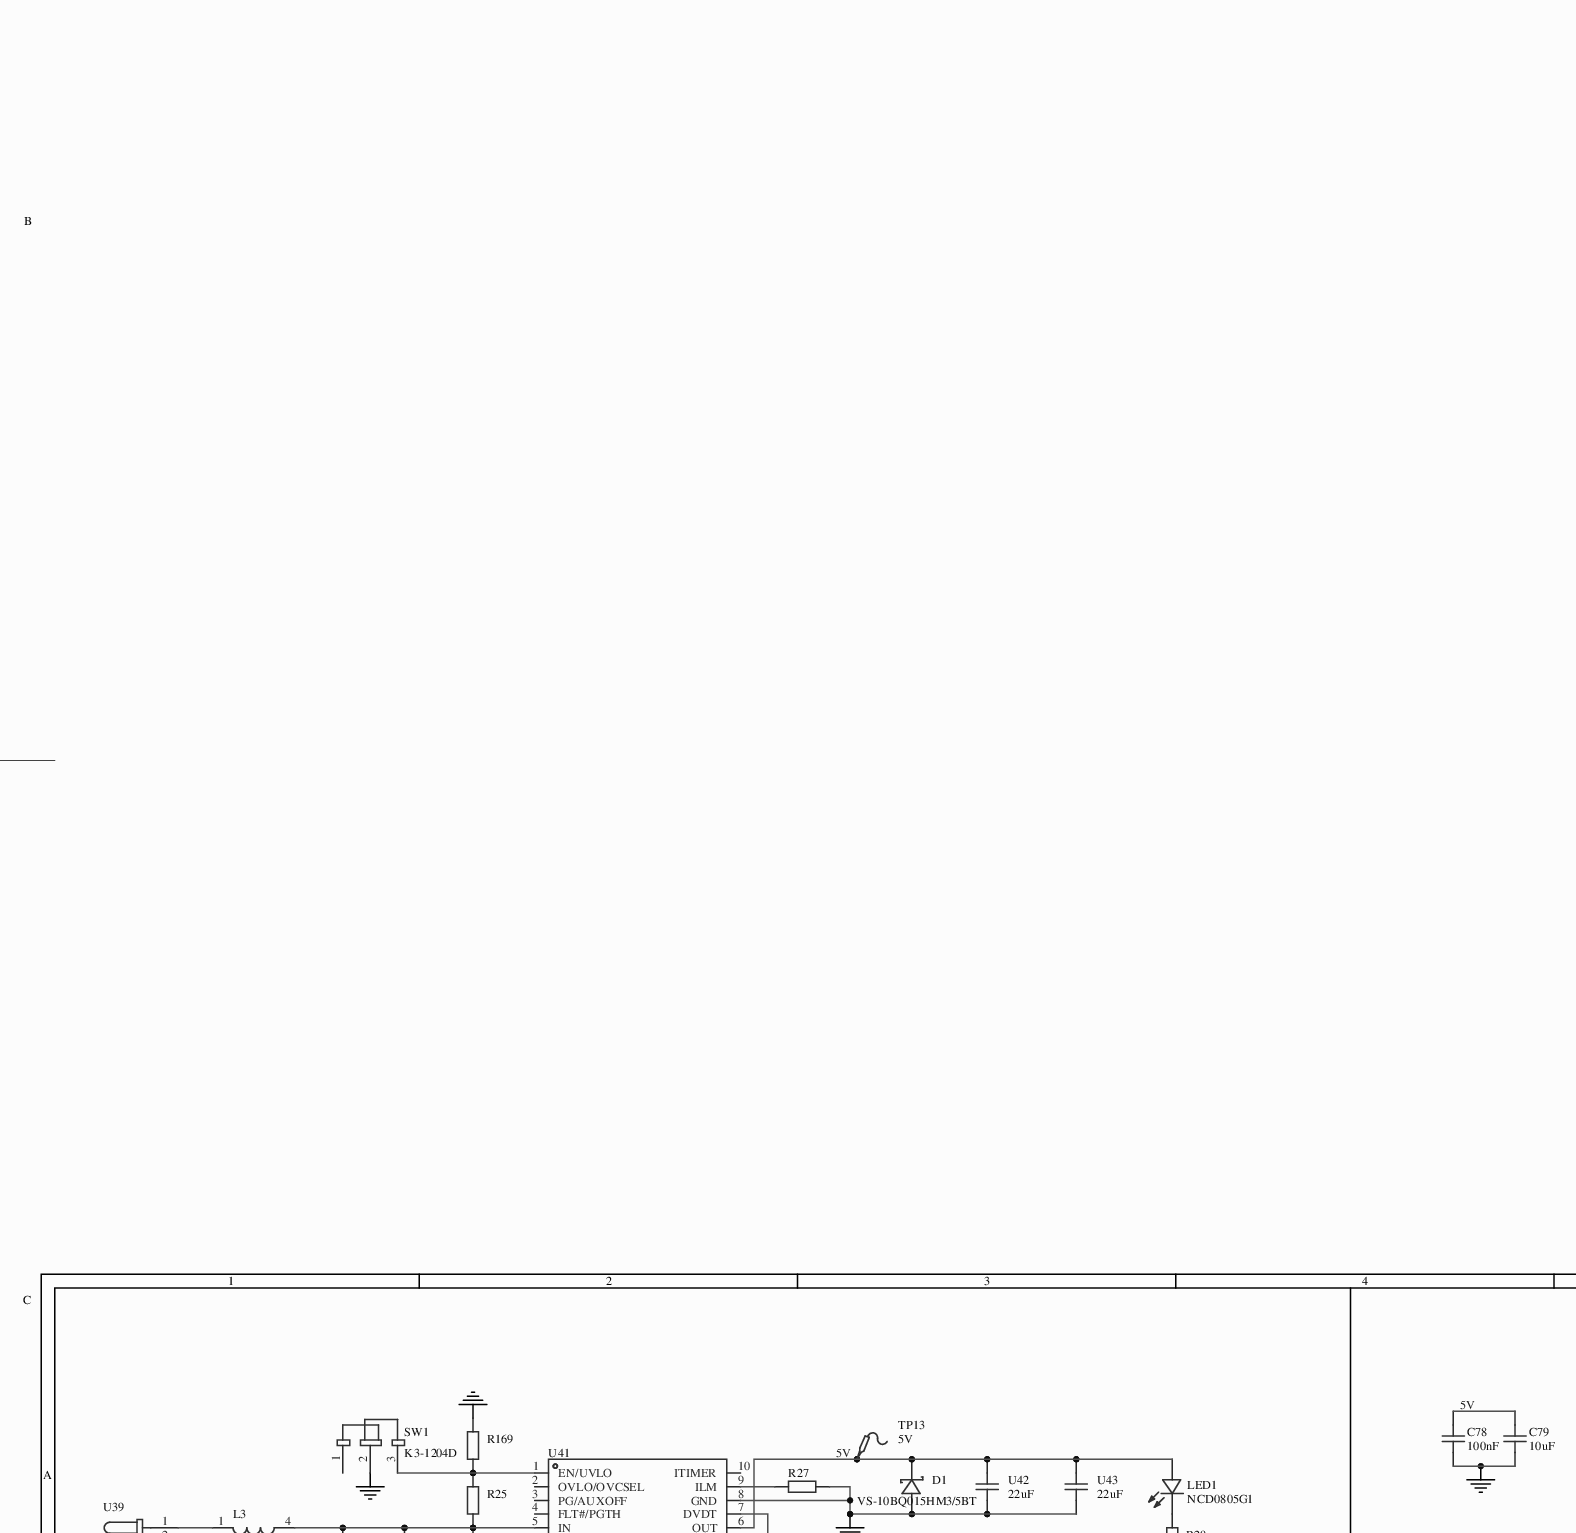
[diagram p0: MISC82799-2.schdoc, centre column 1 of 4]
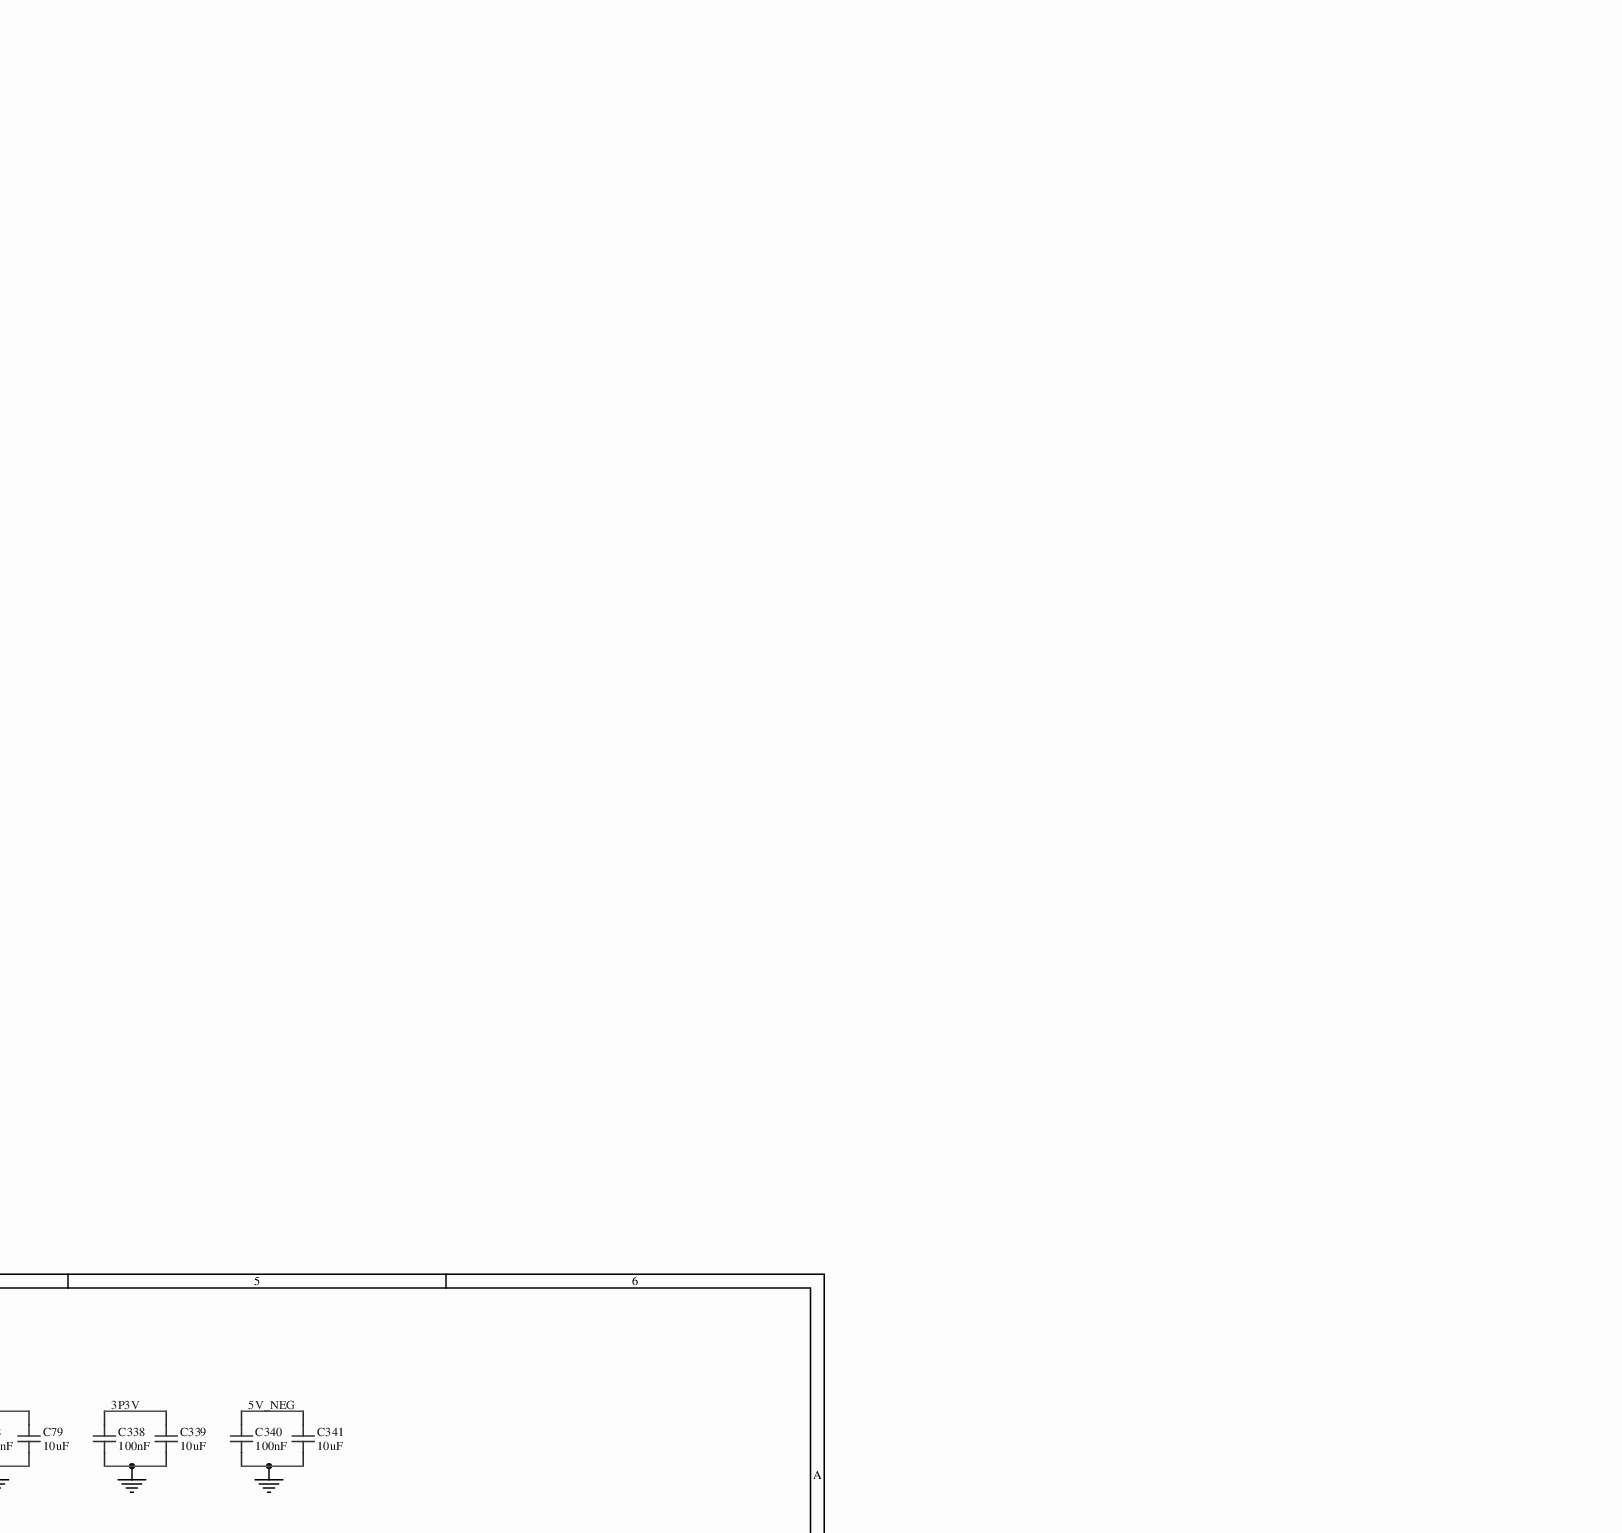
[diagram p1: MISC82799-2.schdoc, centre column 2 of 4]
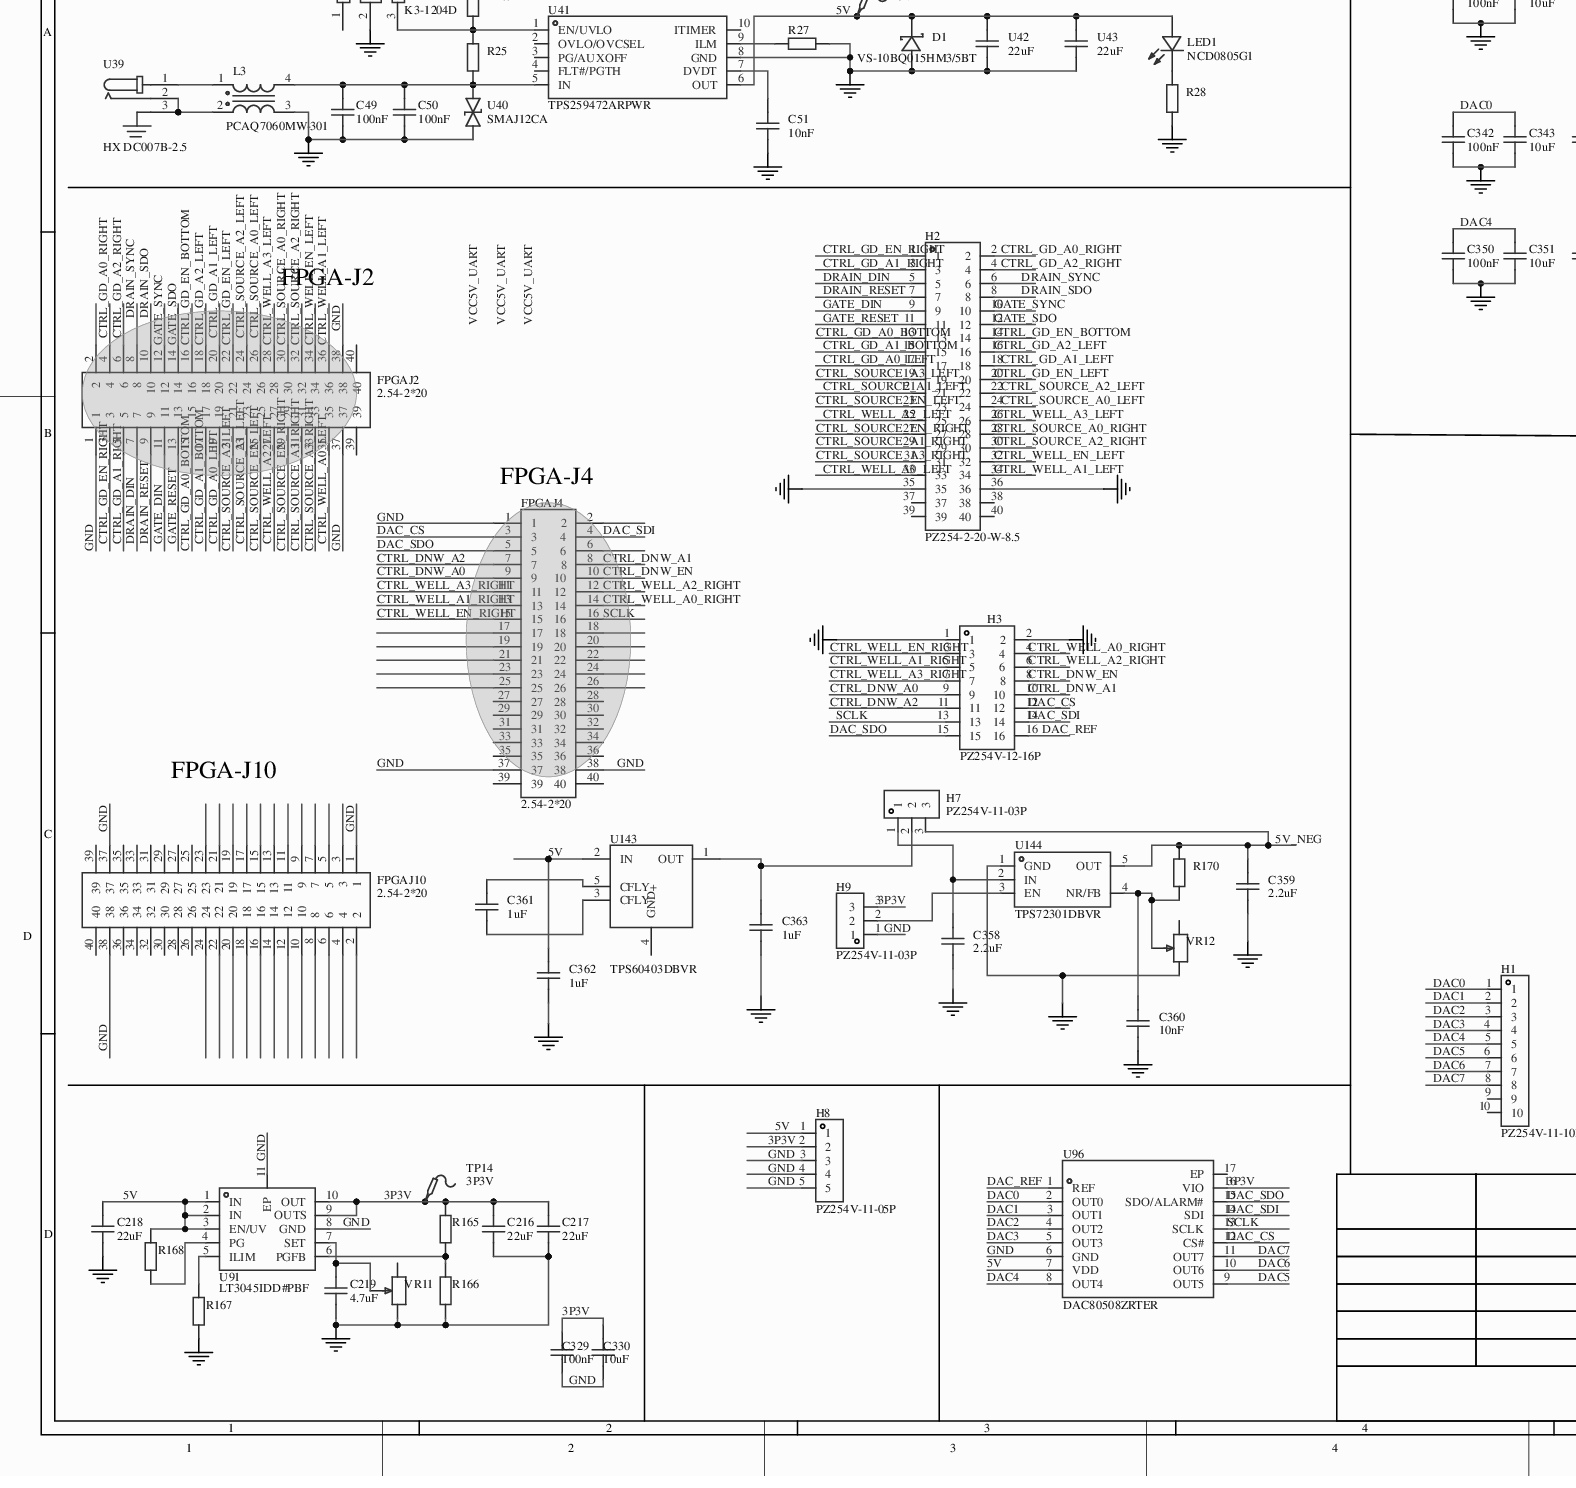
[diagram p2: MISC82799-2.schdoc, bottom column 1 of 4]
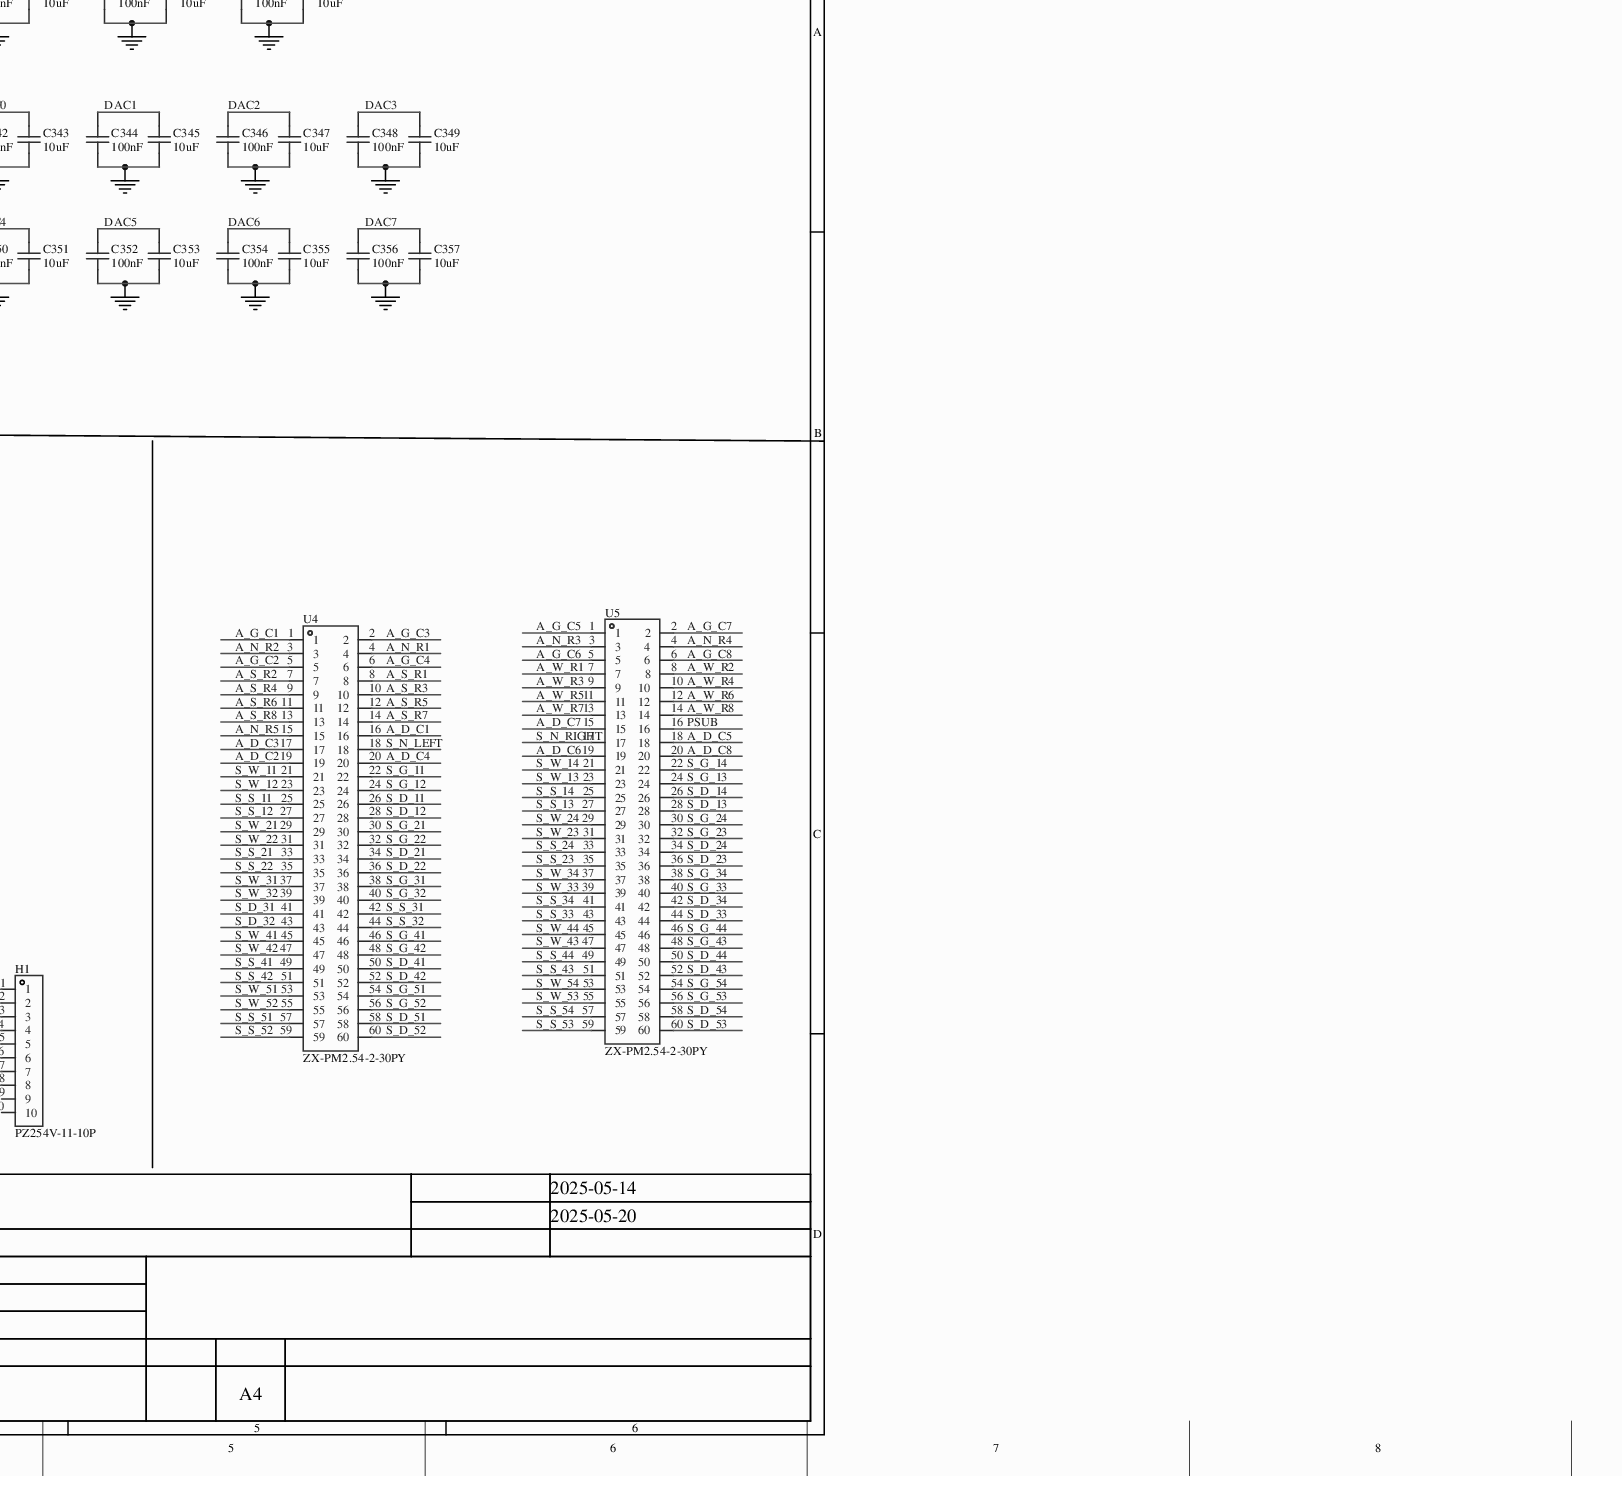
[diagram p3: MISC82799-2.schdoc, bottom column 2 of 4]
# Altium project MISC82799-9.PrjPCB (part 1 of 3)
2 sheets, 95 parts. Net scope: global (net labels, ports and power ports of the same name join across sheets).
Board file: MISC82799.PcbDoc
Sheets:
  MISC82799-2.schdoc
  MISC82799-4.schdoc

## Sheet MISC82799-2.schdoc
size A0; Name: MISC82799; @Page No: 1; @Page Count: 2; @Schematic Name: MISC82799; @Project Name: MISC82799; @Board Name: MISC82799; @Update Date: 2025-05-26; @Create Time: 16:47:34; @Update Time: 16:47:50; @Create Date: 2025-05-26

### Parts
C49  100nF  [C0603]
C50  100nF  [C0603]
C51  10nF  [C0805]
C78  100nF  [C0603]
C79  10uF  [C0603]
C216  22uF  [C0603]
C217  22uF  [C0603]
C218  22uF  [C0603]
C219  4.7uF  [C0603]
C329  100nF  [C0805]
C330  10uF  [C0805]
C338  100nF  [C0603]
C339  10uF  [C0603]
C340  100nF  [C0603]
C341  10uF  [C0603]
C342  100nF  [C0603]
C343  10uF  [C0603]
C344  100nF  [C0603]
C345  10uF  [C0603]
C346  100nF  [C0603]
C347  10uF  [C0603]
C348  100nF  [C0603]
C349  10uF  [C0603]
C350  100nF  [C0603]
C351  10uF  [C0603]
C352  100nF  [C0603]
C353  10uF  [C0603]
C354  100nF  [C0603]
C355  10uF  [C0603]
C356  100nF  [C0603]
C357  10uF  [C0603]
C358  2.2uF  [C0603]
C359  2.2uF  [C0603]
C360  10nF  [C0805]
C361  1uF  [C0603]
C362  1uF  [C0603]
C363  1uF  [C0603]
D1  VS-10BQ015HM3/5BT  [SMB_L4.6-W3.6-LS5.3-RD]
FPGAJ2  2.54-2*20  [HDR-TH_40P-P2.54-V-F-R2-C20-S2.54]
FPGAJ4  2.54-2*20  [HDR-TH_40P-P2.54-V-F-R2-C20-S2.54]
FPGAJ10  2.54-2*20  [HDR-TH_40P-P2.54-V-F-R2-C20-S2.54]
H1  PZ254V-11-10P  [HDR-TH_10P-P2.54-V-M]
H2  PZ254-2-20-W-8.5  [HDR-TH_40P-P2.54-V-F-R2-C20-S2.54]
H3  PZ254V-12-16P  [HDR-TH_16P-P2.54-V-M-R2-C8-S2.54]
H7  PZ254V-11-03P  [HDR-TH_3P-P2.54-V-M]
H8  PZ254V-11-05P  [HDR-TH_5P-P2.54-V-M]
H9  PZ254V-11-03P  [HDR-TH_3P-P2.54-V-M]
L3  PCAQ7060MW-301  [FILTER-SMD_4P-L7.0-W6.0-BL]
LED1  NCD0805G1  [LED0805-R-RD]
R25  (no value)  [R0603]
R27  (no value)  [R0603]
R28  (no value)  [R0603]
R165  (no value)  [R0603]
R166  (no value)  [R0603]
R167  (no value)  [R0603]
R168  (no value)  [R0603]
R169  (no value)  [R0603]
R170  (no value)  [R0603]
SW1  K3-1204D  [SW-TH_K3-1204D]
TP13  5V  [Test-Point-0.5mm]
TP14  3P3V  [Test-Point-0.5mm]
U4  ZX-PM2.54-2-30PY  [HDR-TH_60P-P2.54-V-F-R2-C30-S2.54]
U5  ZX-PM2.54-2-30PY  [HDR-TH_60P-P2.54-V-F-R2-C30-S2.54]
U39  HX DC007B-2.5  [DC-IN-TH_HX-DC007B-2.5]
U40  SMAJ12CA  [SMA_L4.3-W2.7-LS5.1-BI]
U41  TPS259472ARPWR  [VQFN-10_L2.0-W2.0-P0.45-TL]
U42  22uF  [C0805]
U43  22uF  [C0805]
U91  LT3045IDD#PBF  [DFN-10_L3.0-W3.0-P0.50-BL-EP-3]
U96  DAC80508ZRTER  [WQFN-16_L3.0-W3.0-P0.50-TL-EP0.8]
U143  TPS60403DBVR  [SOT-23-5_L3.0-W1.7-P0.95-LS2.8-BR]
U144  TPS72301DBVR  [SOT-23-5_L3.0-W1.7-P0.95-LS2.8-BR]
VR11  (no value)  [RES-ADJ-SMD_3224W]
VR12  (no value)  [RES-ADJ-SMD_3224W]

### Nets
GND: C49.1 C50.1 C51.1 C78.1 C79.1 C216.1 C217.1 C218.1 C219.1 C329.1 C330.1 C338.1 C339.1 C340.1 C341.1 C342.1 C343.1 C344.1 C345.1 C346.1 C347.1 C348.1 C349.1 C350.1 C351.1 C352.1 C353.1 C354.1 C355.1 C356.1 C357.1 C358.1 C359.1 C360.1 C362.1 C363.1 D1.2(A) FPGAJ2.1 FPGAJ2.37 FPGAJ2.38 FPGAJ4.1 FPGAJ4.37 FPGAJ4.38 FPGAJ10.1 FPGAJ10.37 FPGAJ10.38 H2.35 H2.36 H3.1 H3.2 H8.3 H8.4 H8.5 H9.1 L3.3 R27.2 R28.1 R166.1 R167.1 R169.2 SW1.2 U40.1 U41.8(GND) U42.1 U43.1 U91.8(GND) U91.11(EP) U96.6(GND) U144.1(GND) VR11.3 VR12.3
3P3V: C216.2 C217.2 C329.2 C330.2 C338.2 C339.2 H8.2 H9.3 R165.2 TP14.1 U91.9(OUTS) U91.10(OUT) U96.16(VIO)
5V: C78.2 C79.2 C218.2 C362.2 D1.1(C) H8.1 LED1.1(A) R168.2 TP13.1 U41.6(OUT) U42.2 U43.2 U91.1(IN) U91.2(IN) U91.3(EN/UV) U96.7(VDD) U143.2(IN)
5V_NEG: C340.2 C341.2 C359.2 H7.3 R170.2 U144.5(OUT)
A_D_C1: U4.16
A_D_C2: U4.19
A_D_C3: U4.17
A_D_C4: U4.20
A_D_C5: U5.18
A_D_C6: U5.19
A_D_C7: U5.15
A_D_C8: U5.20
A_G_C1: U4.1
A_G_C2: U4.5
A_G_C3: U4.2
A_G_C4: U4.6
A_G_C5: U5.1
A_G_C6: U5.5
A_G_C7: U5.2
A_G_C8: U5.6
A_N_R1: U4.4
A_N_R2: U4.3
A_N_R3: U5.3
A_N_R4: U5.4
A_N_R5: U4.15
A_S_R1: U4.8
A_S_R2: U4.7
A_S_R3: U4.10
A_S_R4: U4.9
A_S_R5: U4.12
A_S_R6: U4.11
A_S_R7: U4.14
A_S_R8: U4.13
A_W_R1: U5.7
A_W_R2: U5.8
A_W_R3: U5.9
A_W_R4: U5.10
A_W_R5: U5.11
A_W_R6: U5.12
A_W_R7: U5.13
A_W_R8: U5.14
CTRL_DNW_A0: FPGAJ4.9 H3.9
CTRL_DNW_A1: FPGAJ4.8 H3.10
CTRL_DNW_A2: FPGAJ4.7 H3.11
CTRL_DNW_EN: FPGAJ4.10 H3.8
CTRL_GD_A0_BOTTOM: FPGAJ2.15 H2.13
CTRL_GD_A0_LEFT: FPGAJ2.19 H2.17
CTRL_GD_A0_RIGHT: FPGAJ2.4 H2.2
CTRL_GD_A1_BOTTOM: FPGAJ2.17 H2.15
CTRL_GD_A1_LEFT: FPGAJ2.20 H2.18
CTRL_GD_A1_RIGHT: FPGAJ2.5 H2.3
CTRL_GD_A2_LEFT: FPGAJ2.18 H2.16
CTRL_GD_A2_RIGHT: FPGAJ2.6 H2.4
CTRL_GD_EN_BOTTOM: FPGAJ2.16 H2.14
CTRL_GD_EN_LEFT: FPGAJ2.22 H2.20
CTRL_GD_EN_RIGHT: FPGAJ2.3 H2.1
CTRL_SOURCE_A0_LEFT: FPGAJ2.26 H2.24
CTRL_SOURCE_A0_RIGHT: FPGAJ2.30 H2.28
CTRL_SOURCE_A1_LEFT: FPGAJ2.23 H2.21
CTRL_SOURCE_A1_RIGHT: FPGAJ2.31 H2.29
CTRL_SOURCE_A2_LEFT: FPGAJ2.24 H2.22
CTRL_SOURCE_A2_RIGHT: FPGAJ2.32 H2.30
CTRL_SOURCE_A3_LEFT: FPGAJ2.21 H2.19
CTRL_SOURCE_A3_RIGHT: FPGAJ2.33 H2.31
CTRL_SOURCE_EN_LEFT: FPGAJ2.25 H2.23
CTRL_SOURCE_EN_RIGHT: FPGAJ2.29 H2.27
CTRL_WELL_A0_LEFT: FPGAJ2.35 H2.33
CTRL_WELL_A0_RIGHT: FPGAJ4.14 H3.4
CTRL_WELL_A1_LEFT: FPGAJ2.36 H2.34
CTRL_WELL_A1_RIGHT: FPGAJ4.13 H3.5
CTRL_WELL_A2_LEFT: FPGAJ2.27 H2.25
CTRL_WELL_A2_RIGHT: FPGAJ4.12 H3.6
CTRL_WELL_A3_LEFT: FPGAJ2.28 H2.26
CTRL_WELL_A3_RIGHT: FPGAJ4.11 H3.7
CTRL_WELL_EN_LEFT: FPGAJ2.34 H2.32
CTRL_WELL_EN_RIGHT: FPGAJ4.15 H3.3
DAC0: C342.2 C343.2 H1.1 U96.2(OUT0)
DAC1: C344.2 C345.2 H1.2 U96.3(OUT1)
DAC2: C346.2 C347.2 H1.3 U96.4(OUT2)
DAC3: C348.2 C349.2 H1.4 U96.5(OUT3)
DAC4: C350.2 C351.2 H1.5 U96.8(OUT4)
DAC5: C352.2 C353.2 H1.6 U96.9(OUT5)
DAC6: C354.2 C355.2 H1.7 U96.10(OUT6)
DAC7: C356.2 C357.2 H1.8 U96.11(OUT7)
DAC_CS: FPGAJ4.3 H3.12 U96.12(CS#)
DAC_REF: H3.16 U96.1(REF)
DAC_SDI: FPGAJ4.4 H3.14 U96.14(SDI)
DAC_SDO: FPGAJ4.5 H3.15 U96.15(SDO/ALARM#)
DRAIN_DIN: FPGAJ2.7 H2.5
DRAIN_RESET: FPGAJ2.9 H2.7
DRAIN_SDO: FPGAJ2.10 H2.8
DRAIN_SYNC: FPGAJ2.8 H2.6
GATE_DIN: FPGAJ2.11 H2.9
GATE_RESET: FPGAJ2.13 H2.11
GATE_SDO: FPGAJ2.14 H2.12
GATE_SYNC: FPGAJ2.12 H2.10
PSUB: U5.16
S_D_11: U4.26
S_D_12: U4.28
S_D_13: U5.28
S_D_14: U5.26
S_D_21: U4.34
S_D_22: U4.36
S_D_23: U5.36
S_D_24: U5.34
S_D_31: U4.41
S_D_32: U4.43
S_D_33: U5.44
S_D_34: U5.42
S_D_41: U4.50
S_D_42: U4.52
S_D_43: U5.52
S_D_44: U5.50
S_D_51: U4.58
S_D_52: U4.60
S_D_53: U5.60
S_D_54: U5.58
S_G_11: U4.22
S_G_12: U4.24
S_G_13: U5.24
S_G_14: U5.22
S_G_21: U4.30
S_G_22: U4.32
S_G_23: U5.32
S_G_24: U5.30
S_G_31: U4.38
S_G_32: U4.40
S_G_33: U5.40
S_G_34: U5.38
S_G_41: U4.46
S_G_42: U4.48
S_G_43: U5.48
S_G_44: U5.46
S_G_51: U4.54
S_G_52: U4.56
S_G_53: U5.56
S_G_54: U5.54
S_N_LEFT: U4.18
S_N_RIGHT: U5.17
S_S_11: U4.25
S_S_12: U4.27
S_S_13: U5.27
S_S_14: U5.25
S_S_21: U4.33
S_S_22: U4.35
S_S_23: U5.35
S_S_24: U5.33
S_S_31: U4.42
S_S_32: U4.44
S_S_33: U5.43
S_S_34: U5.41
S_S_41: U4.49
S_S_42: U4.51
S_S_43: U5.51
S_S_44: U5.49
S_S_51: U4.57
S_S_52: U4.59
S_S_53: U5.59
S_S_54: U5.57
S_W_11: U4.21
S_W_12: U4.23
S_W_13: U5.23
S_W_14: U5.21
S_W_21: U4.29
S_W_22: U4.31
S_W_23: U5.31
S_W_24: U5.29
S_W_31: U4.37
S_W_32: U4.39
S_W_33: U5.39
S_W_34: U5.37
S_W_41: U4.45
S_W_42: U4.47
S_W_43: U5.47
S_W_44: U5.45
S_W_51: U4.53
S_W_52: U4.55
S_W_53: U5.55
S_W_54: U5.53
SCLK: FPGAJ4.16 H3.13 U96.13(SCLK)
NetC49_2: C49.2 C50.2 L3.4 R25.1 U40.2 U41.5(IN)
NetC51_2: C51.2 U41.7(DVDT)
NetC219_2: C219.2 U91.7(SET) VR11.2
NetC358_2: C358.2 H7.1 U144.2(IN)
NetC360_2: C360.2 R170.1 U144.4(NR/FB) VR12.2
NetC361_1: C361.1 U143.3(CFLY-)
NetC361_2: C361.2 U143.5(CFLY+)
NetC363_2: C363.2 H7.2 U143.1(OUT)
NetH9_2: H9.2 U144.3(EN)
NetL3_1: L3.1 U39.1
NetL3_2: L3.2 U39.2 U39.3
NetLED1_2: LED1.2(K) R28.2
NetR25_2: R25.2 R169.1 SW1.3 U41.1(EN/UVLO)
NetR27_1: R27.1 U41.9(ILM)
NetR165_1: R165.1 R166.2 U91.6(PGFB)
NetR167_2: R167.2 U91.5(ILIM)
NetR168_1: R168.1 U91.4(PG)

Not connected (* = marked no-connect by the designer): FPGAJ2 2 39 40; FPGAJ4 2 6 17 18 19 20 21 22 23 24 25 26 27 28 29 30 31 32 33 34 35 36 39 40; FPGAJ10 2 3 4 5 6 7 8 9 10 11 12 13 14 15 16 17 18 19 20 21 22 23 24 25 26 27 28 29 30 31 32 33 34 35 36 39 40; H1 9 10; H2 37 38 39 40; SW1 1; U41 2(OVLO/OVCSEL) 3(PG/AUXOFF) 4(FLT#/PGTH) 10(ITIMER); U96 17(EP); U143 4(GND); VR11 1; VR12 1

### Notes on the sheet
- FPGA-J2
- (near FPGAJ4) FPGA-J4
- FPGA-J10
- Labels drawn without touching a wire or pin: VCC5V_UART
- 1
- 2
- 3
- 4
- 5
- 6
- A
- B
- C
- D
- 2025-05-14
- 2025-05-20
- A4

### Library data of the parts
C49 C50 = CL10B104KA8NNNC: Add into BOM: yes; Voltage Rated: 25V; Temperature Coefficient: X7R; Symbol: 100nF; Device: CL10B104KA8NNNC; Supplier Part: C1590; Manufacturer Part: CL10B104KA8NNNC; Supplier Footprint: 0603; JLCPCB Part Class: Extended Part; Datasheet: https://example.com/upload/public/pdf/source/20160218/1457707763339.pdf; Supplier: LCSC; Convert to PCB: yes; Value: 100nF
C51 C360 = CL21B103KBANNNC: Add into BOM: yes; Voltage Rated: 50V; Temperature Coefficient: X7R; Device: CL21B103KBANNNC; Supplier Part: C1710; Manufacturer Part: CL21B103KBANNNC; Supplier Footprint: 0805; JLCPCB Part Class: Basic Part; Datasheet: https://example.com/upload/public/pdf/source/20160218/1457707763339.pdf; Supplier: LCSC; Convert to PCB: yes; Value: 10nF
  C51: Symbol: 10nF
  C360: Symbol: CL21B103KBANNNC; Origin Footprint: C0805
C78 C338 C340 C342 C344 C346 C348 C350 C352 C354 C356 = CL10B104JB8NNNC: Add into BOM: yes; Voltage Rated: 50V; Temperature Coefficient: X7R; Symbol: 100nF; Device: CL10B104JB8NNNC; Supplier Part: C24452; Manufacturer Part: CL10B104JB8NNNC; Supplier Footprint: 0603; JLCPCB Part Class: Extended Part; Datasheet: https://example.com/upload/public/pdf/source/20160218/1457707763339.pdf; Supplier: LCSC; Convert to PCB: yes; Value: 100nF
C79 C339 C341 C343 C345 C347 C349 C351 C353 C355 C357 = CL10A106KO8NQNC: Add into BOM: yes; Voltage Rated: 16V; Temperature Coefficient: X5R; Symbol: 10uF; Device: CL10A106KO8NQNC; Supplier Part: C962136; Manufacturer Part: CL10A106KO8NQNC; Supplier Footprint: 0603; JLCPCB Part Class: Extended Part; Datasheet: https://example.com/upload/public/pdf/source/20160218/1457707763339.pdf; Supplier: LCSC; Convert to PCB: yes; Value: 10uF
C216-C218 = CL10A226MO7JZNC: Add into BOM: yes; Voltage Rated: 16V; Temperature Coefficient: X5R; Symbol: 22uF; Device: CL10A226MO7JZNC; Supplier Part: C2762594; Manufacturer Part: CL10A226MO7JZNC; Supplier Footprint: 0603; JLCPCB Part Class: Extended Part; Datasheet: https://example.com/upload/public/pdf/source/20220811/0832C3B1C642040B023B7A6186895861.pdf; Supplier: LCSC; Convert to PCB: yes; Value: 22uF
C219 = CL10A475KA8NQNC: Add into BOM: yes; Voltage Rated: 25V; Temperature Coefficient: X5R; Symbol: 4.7uF; Device: CL10A475KA8NQNC; Supplier Part: C69335; Manufacturer Part: CL10A475KA8NQNC; Supplier Footprint: 0603; JLCPCB Part Class: Extended Part; Datasheet: https://example.com/upload/public/pdf/source/20161108/1478586410580.pdf; Supplier: LCSC; Convert to PCB: yes; Value: 4.7uF
C329 = CL21B104KCFNNNE: Add into BOM: yes; Voltage Rated: 100V; Temperature Coefficient: X7R; Symbol: 100nF; Device: CL21B104KCFNNNE; Supplier Part: C28233; Manufacturer Part: CL21B104KCFNNNE; Supplier Footprint: 0805; JLCPCB Part Class: Basic Part; Datasheet: https://example.com/upload/public/pdf/source/20160218/1457707763339.pdf; Supplier: LCSC; Convert to PCB: yes; Value: 100nF